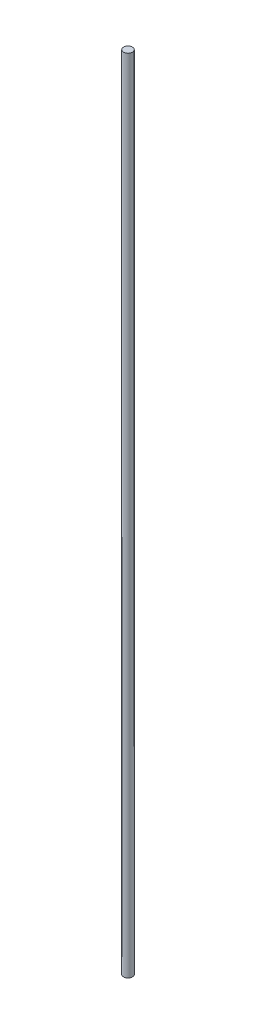
from build123d import *

# Parameters (mm, degrees)
SKETCH1_W = 0.5
SKETCH1_H = 90


with BuildPart() as part:
    # Sketch1 → Revolve1 (revolve)
    with BuildSketch(Plane.XY, mode=Mode.PRIVATE) as revolve1_sk:
        with Locations((-0.25, 45)):
            Rectangle(SKETCH1_W, SKETCH1_H)
    revolve(revolve1_sk.sketch.rotate(Axis((0, -6.441627678, 0), (0, 1, 0)), 270), axis=Axis((0, -6.441627678, 0), (0, 1, 0)))


solid = part.part
